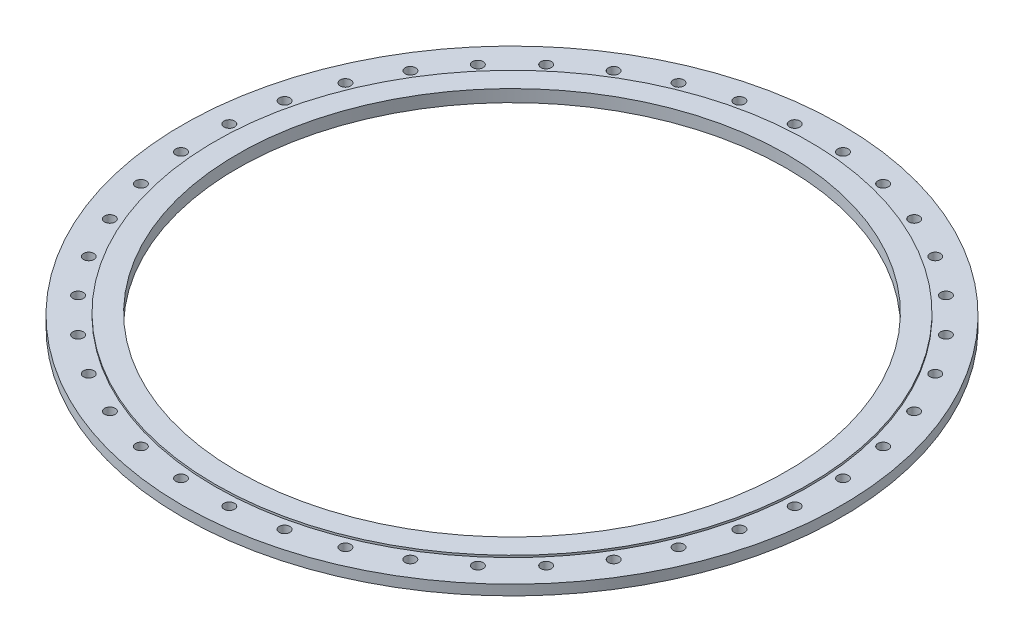
SolidWorks part; units mm, degrees
material "Q235B"
ref_plane "前视基准面" through (0, 0, 0) normal (0, 0, 1) x (1, 0, 0)
ref_plane "上视基准面" through (0, 0, 0) normal (0, 1, 0) x (1, 0, 0)
ref_plane "右视基准面" through (0, 0, 0) normal (1, 0, 0) x (0, 0, -1)
sketch "草图1" plane through (0, 0, 0) normal (0, 1, 0) x (1, 0, 0)
  circle A0 centre (0, 0) radius 810
  circle A1 centre (0, 0) radius 675 construction
  dimension "D1" = 1620
  dimension "D2" = 1350
extrude "凸台-拉伸1" add sketch "草图1" along normal blind 25
sketch "草图2" plane through (0, 25, 0) normal (0, 1, 0) x (1, 0, 0)
  circle A0 centre (0, 0) radius 730
  dimension "D2" = 1460
extrude "凸台-拉伸2" add sketch "草图2" along normal blind 5
sketch "草图3" plane through (0, 30, 0) normal (0, 1, 0) x (1, 0, 0)
  line L1 (130, -662.3632) -> (-130, -662.3632)
  line L2 (130, -662.3632) -> (130, 662.3632)
  line L3 (130, 662.3632) -> (-130, 662.3632)
  line L4 (-130, -662.3632) -> (-130, 662.3632)
  line L5 (130, -662.3632) -> (-130, 662.3632) construction
  line L6 (130, 662.3632) -> (-130, -662.3632) construction
  circle A0 centre (0, 0) radius 675
  circle A1 centre (0, 0) radius 75
  dimension "D1" = 1350
  dimension "D3" = 150
  dimension "D2" = 260
extrude "切除-拉伸1" cut sketch "草图3" against normal up to next contours L2 A0 | L4 A0 | A1
sketch "草图4" plane through (0, 30, 0) normal (0, 1, 0) x (1, 0, 0)
  circle A0 centre (0, 0) radius 110
  dimension "D1" = 220
extrude "切除-拉伸2" cut sketch "草图4" against normal blind 5
hole_wizard "M8 螺纹孔1" positions "草图5" profile "草图6" tap size "M8" standard "GB" end condition up to next
sketch "草图5" plane through (0, 25, 0) normal (0, 1, 0) x (1, 0, 0)
  line L0 (0, 0) -> (0, 85)
  circle A0 centre (0, 0) radius 85 construction
  point P0 (0, 85)
  point P15 (85, 0)
  point P16 (0, -85)
  point P17 (-85, 0)
  dimension "D1" = 170
  dimension "D2" = 4
sketch "草图6" plane through (0, 25, -85) normal (1, 0, 0) x (0, 0, 1)
  line L0 (0, 0) -> (0, 25)
  line L1 (0, 25) -> (3.4, 25)
  line L2 (3.4, 25) -> (3.4, 0)
  line L5 (3.4, 0) -> (0, 0)
  line L11 (0, -6.35) -> (0, 107.95) construction
  dimension "通孔螺纹孔钻头直径" = 6.8
  dimension "通孔螺纹孔钻头深度" = 25
cosmetic thread "孔螺蚊线1" parameters "D2"=8
cosmetic thread "孔螺蚊线2" parameters "D2"=8
cosmetic thread "孔螺蚊线3" parameters "D2"=8
cosmetic thread "孔螺蚊线4" parameters "D2"=8
hole_wizard "Ø25.5 (25.5) 直径孔1" positions "草图9" profile "草图8" hole size "Ø25.5" standard "GB" end condition up to next
sketch "草图9" plane through (0, 25, 0) normal (0, 1, 0) x (1, 0, 0)
  line L0 (0, 0) -> (0, 756.5) construction
  circle A0 centre (0, 0) radius 756.5 construction
  point P0 (-59.3543, 754.168)
  point P14 (59.3543, 754.168)
  point P15 (176.6014, 735.5978)
  point P16 (289.5, 698.9149)
  point P17 (395.2702, 645.0223)
  point P18 (491.3074, 575.2471)
  point P19 (575.2471, 491.3074)
  point P20 (645.0223, 395.2702)
  point P21 (698.9149, 289.5)
  point P22 (735.5978, 176.6014)
  point P23 (754.168, 59.3543)
  point P24 (754.168, -59.3543)
  point P25 (735.5978, -176.6014)
  point P26 (698.9149, -289.5)
  point P27 (645.0223, -395.2702)
  point P28 (575.2471, -491.3074)
  point P29 (491.3074, -575.2471)
  point P30 (395.2702, -645.0223)
  point P31 (289.5, -698.9149)
  point P32 (176.6014, -735.5978)
  point P33 (59.3543, -754.168)
  point P34 (-59.3543, -754.168)
  point P35 (-176.6014, -735.5978)
  point P36 (-289.5, -698.9149)
  point P37 (-395.2702, -645.0223)
  point P38 (-491.3074, -575.2471)
  point P39 (-575.2471, -491.3074)
  point P40 (-645.0223, -395.2702)
  point P41 (-698.9149, -289.5)
  point P42 (-735.5978, -176.6014)
  point P43 (-754.168, -59.3543)
  point P44 (-754.168, 59.3543)
  point P45 (-735.5978, 176.6014)
  point P46 (-698.9149, 289.5)
  point P47 (-645.0223, 395.2702)
  point P48 (-575.2471, 491.3074)
  point P49 (-491.3074, 575.2471)
  point P50 (-395.2702, 645.0223)
  point P51 (-289.5, 698.9149)
  point P52 (-176.6014, 735.5978)
  dimension "D1" = 1513
  dimension "D2" = 40
sketch "草图8" plane through (-59.3543, 25, -754.168) normal (1, 0, 0) x (0, 0, 1)
  line L0 (0, 0) -> (0, 25)
  line L1 (0, 25) -> (13, 25)
  line L2 (13, 25) -> (13, 0)
  line L5 (13, 0) -> (0, 0)
  line L11 (0, -6.35) -> (0, 107.95) construction
  dimension "通孔孔直径" = 26
  dimension "通孔孔深度" = 25
sketch "草图10" plane through (0, 30, 0) normal (0, 1, 0) x (1, 0, 0)
  circle A0 centre (0, 0) radius 675
extrude "切除-拉伸3" cut sketch "草图10" against normal through all both and the other way through all
